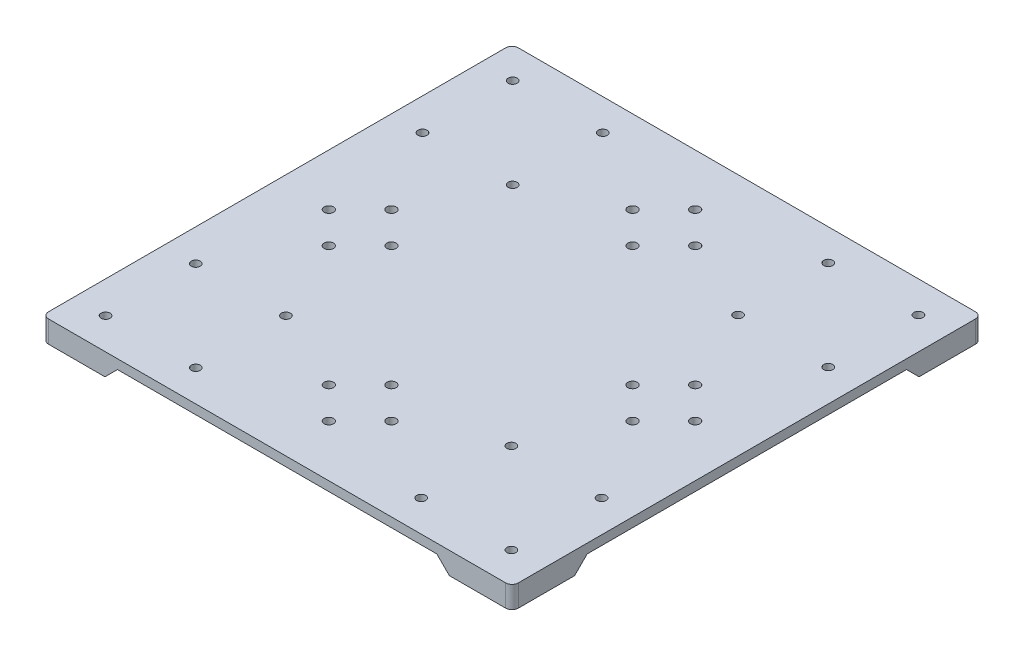
from build123d import *

# Parameters (mm, degrees)
SKETCH1_W           = 150
SKETCH1_H           = 150
BOSS_EXTRUDE1_DEPTH = 3
SKETCH2_R           = 1.44
CUT_EXTRUDE1_DEPTH  = 107.108435103
SKETCH3_R           = 1.5
CUT_EXTRUDE2_DEPTH  = 107.108435103
FILLET1_R           = 2
SKETCH4_W           = 144
SKETCH4_H           = 144
BOSS_EXTRUDE2_DEPTH = 4
CUT_EXTRUDE3_DEPTH  = 168.752794314
CUT_EXTRUDE4_DEPTH  = 168.752794314


with BuildPart() as part:
    # Sketch1 → Boss-Extrude1 (new body)
    with BuildSketch(Plane(origin=(0, 0, 0), x_dir=(1, 0, 0), z_dir=(0, 1, 0))):
        Rectangle(SKETCH1_W, SKETCH1_H)
    extrude(amount=BOSS_EXTRUDE1_DEPTH)

    # Sketch2 → Cut-Extrude1 (cut, through all)
    with BuildSketch(Plane(origin=(0, 3, 0), x_dir=(1, 0, 0), z_dir=(0, 1, 0))):
        with Locations(Location((-64.8, 65, 0), (0, 0, 270))):
            Circle(SKETCH2_R)
        with Locations(Location((-36, 65, 0), (0, 0, 270))):
            Circle(SKETCH2_R)
        with Locations(Location((-64.8, 36.2, 0), (0, 0, 270))):
            Circle(SKETCH2_R)
        with Locations(Location((-36, 36.2, 0), (0, 0, 270))):
            Circle(SKETCH2_R)
        with Locations(Location((36, 65, 0), (0, 0, 90))):
            Circle(SKETCH2_R)
        with Locations(Location((64.8, 65, 0), (0, 0, 90))):
            Circle(SKETCH2_R)
        with Locations(Location((64.8, 36.2, 0), (0, 0, 90))):
            Circle(SKETCH2_R)
        with Locations(Location((36, 36.2, 0), (0, 0, 90))):
            Circle(SKETCH2_R)
        with Locations(Location((-64.8, -36.2, 0), (0, 0, 90))):
            Circle(SKETCH2_R)
        with Locations(Location((-64.8, -65, 0), (0, 0, 90))):
            Circle(SKETCH2_R)
        with Locations(Location((-36, -65, 0), (0, 0, 90))):
            Circle(SKETCH2_R)
        with Locations(Location((-36, -36.2, 0), (0, 0, 90))):
            Circle(SKETCH2_R)
        with Locations(Location((64.8, -65, 0), (0, 0, 270))):
            Circle(SKETCH2_R)
        with Locations(Location((36, -65, 0), (0, 0, 270))):
            Circle(SKETCH2_R)
        with Locations(Location((36, -36.2, 0), (0, 0, 270))):
            Circle(SKETCH2_R)
        with Locations(Location((64.8, -36.2, 0), (0, 0, 270))):
            Circle(SKETCH2_R)
    extrude(amount=-CUT_EXTRUDE1_DEPTH, mode=Mode.SUBTRACT)

    # Sketch3 → Cut-Extrude2 (cut, through all)
    with BuildSketch(Plane(origin=(0, 3, 0), x_dir=(1, 0, 0), z_dir=(0, 1, 0))):
        with Locations(Location((-38.5, 0, 0), (0, 0, 270))):
            Circle(SKETCH3_R)
        with Locations(Location((-48.5, 10, 0), (0, 0, 270))):
            Circle(SKETCH3_R)
        with Locations(Location((-58.5, 0, 0), (0, 0, 270))):
            Circle(SKETCH3_R)
        with Locations(Location((-48.5, -10, 0), (0, 0, 270))):
            Circle(SKETCH3_R)
        with Locations(Location((-10, -48.5, 0), (0, 0, 270))):
            Circle(SKETCH3_R)
        with Locations(Location((0, -58.5, 0), (0, 0, 270))):
            Circle(SKETCH3_R)
        with Locations(Location((10, -48.5, 0), (0, 0, 270))):
            Circle(SKETCH3_R)
        with Locations(Location((0, -38.5, 0), (0, 0, 270))):
            Circle(SKETCH3_R)
        with Locations(Location((58.5, 0, 0), (0, 0, 270))):
            Circle(SKETCH3_R)
        with Locations(Location((48.5, 10, 0), (0, 0, 270))):
            Circle(SKETCH3_R)
        with Locations(Location((38.5, 0, 0), (0, 0, 270))):
            Circle(SKETCH3_R)
        with Locations(Location((0, 38.5, 0), (0, 0, 270))):
            Circle(SKETCH3_R)
        with Locations(Location((10, 48.5, 0), (0, 0, 270))):
            Circle(SKETCH3_R)
        with Locations(Location((0, 58.5, 0), (0, 0, 270))):
            Circle(SKETCH3_R)
        with Locations(Location((-10, 48.5, 0), (0, 0, 270))):
            Circle(SKETCH3_R)
        with Locations(Location((48.5, -10, 0), (0, 0, 270))):
            Circle(SKETCH3_R)
    extrude(amount=-CUT_EXTRUDE2_DEPTH, mode=Mode.SUBTRACT)

    # Fillet1
    fillet1_edges = [part.edges().sort_by_distance(p)[0] for p in [
        (75, 1.5, 75),
        (-75, 1.5, 75),
        (-75, 1.5, -75),
        (75, 1.5, -75),
    ]]
    fillet(fillet1_edges, radius=FILLET1_R)

    # Sketch4 → Boss-Extrude2 (add)
    with BuildSketch(Plane.XZ):
        with BuildLine():
            Line((73, -75), (-73, -75))
            ThreePointArc((-73, -75), (-74.414213562, -74.414213562), (-75, -73))
            Line((-75, -73), (-75, 73))
            ThreePointArc((-75, 73), (-74.414213562, 74.414213562), (-73, 75))
            Line((-73, 75), (73, 75))
            ThreePointArc((73, 75), (74.414213562, 74.414213562), (75, 73))
            Line((75, 73), (75, -73))
            ThreePointArc((75, -73), (74.414213562, -74.414213562), (73, -75))
        make_face()
        Rectangle(SKETCH4_W, SKETCH4_H, mode=Mode.SUBTRACT)
    extrude(amount=BOSS_EXTRUDE2_DEPTH)

    # Sketch5 → Cut-Extrude3 (cut, through all)
    with BuildSketch(Plane.XY.offset(75)):
        Polygon((-55, -4), (-51, 0), (51, 0), (55, -4), align=None)
    extrude(amount=-CUT_EXTRUDE3_DEPTH, mode=Mode.SUBTRACT)

    # Sketch6 → Cut-Extrude4 (cut, through all)
    with BuildSketch(Plane.ZY.offset(75)):
        Polygon((-55, -4), (-51, 0), (51, 0), (55, -4), align=None)
    extrude(amount=-CUT_EXTRUDE4_DEPTH, mode=Mode.SUBTRACT)


solid = part.part
